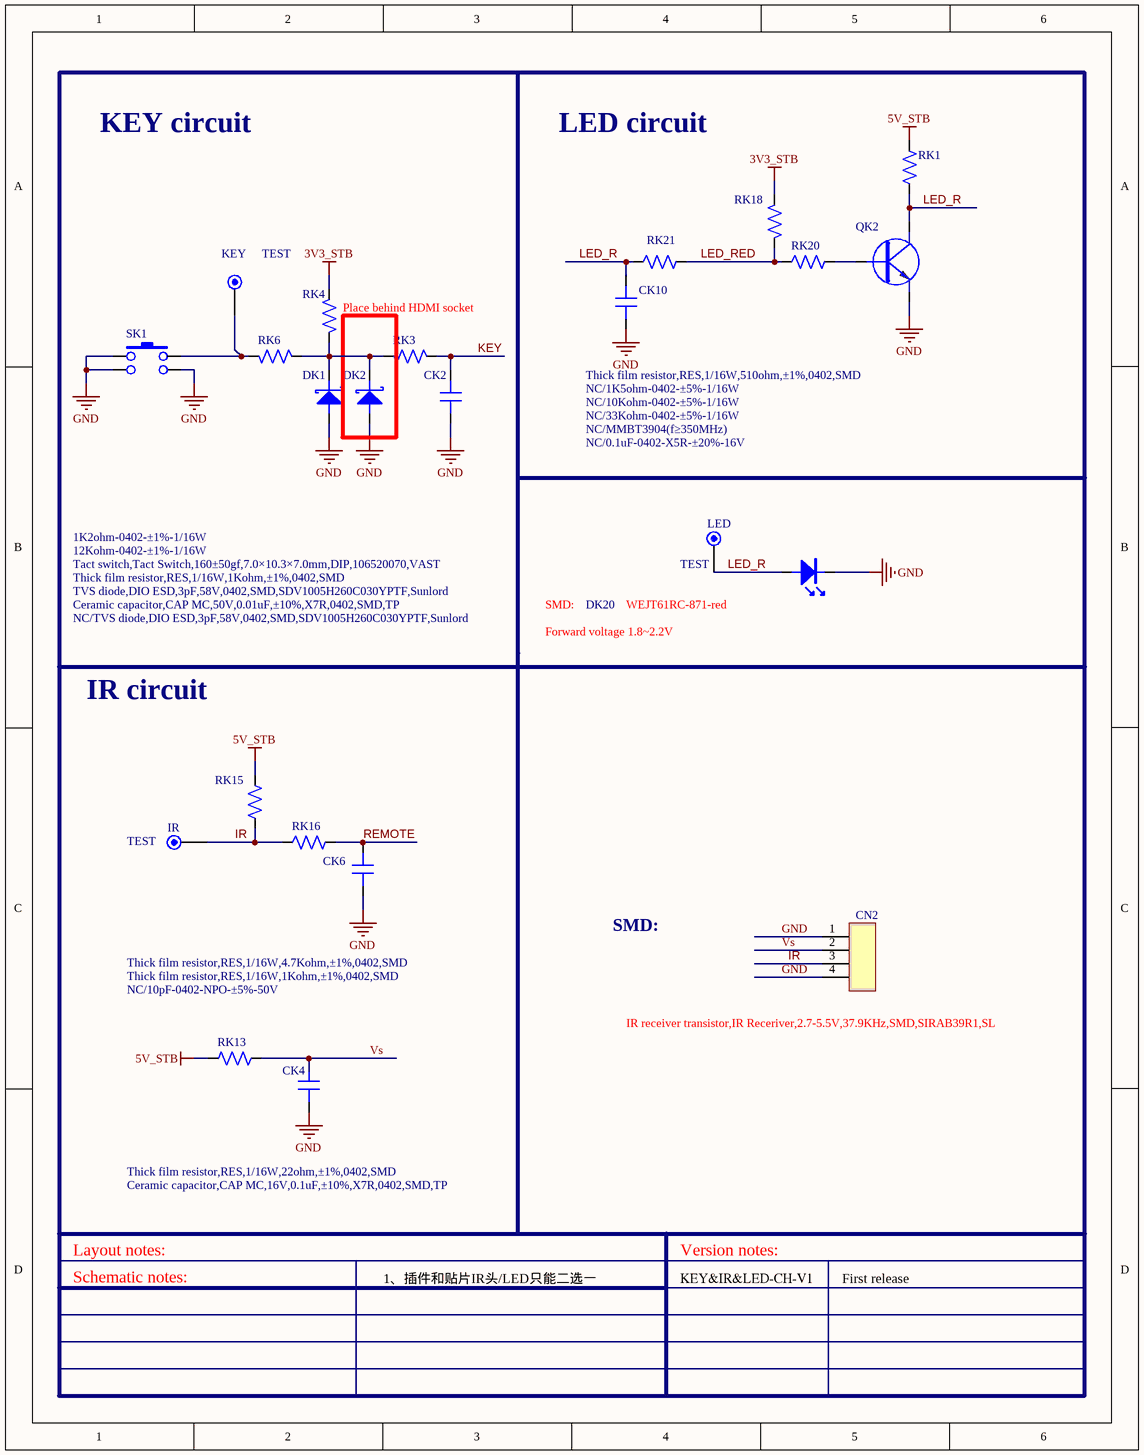
[diagram p0: MISC86383-17.SchDoc]
# Altium schematic sheet MISC86383-17.SchDoc
size 213 x 271 mm

## Parts
CK2  Ceramic capacitor,CAP MC,50V,0.01uF,±10%,X7R,0402,SMD,TP  [C0402]
CK4  Ceramic capacitor,CAP MC,16V,0.1uF,±10%,X7R,0402,SMD,TP  [C0402]
CK6  NC/10pF-0402-NPO-±5%-50V  [C0402]
CK10  NC/0.1uF-0402-X5R-±20%-16V  [C0402]
CN2  IR receiver transistor,IR Receriver,2.7-5.5V,37.9KHz,SMD,SIRAB39R1,SL  [REMOTE-HS-1]
DK1  TVS diode,DIO ESD,3pF,58V,0402,SMD,SDV1005H260C030YPTF,Sunlord  [DIODE-S0402]
DK2  NC/TVS diode,DIO ESD,3pF,58V,0402,SMD,SDV1005H260C030YPTF,Sunlord  [DIODE-S0402]
DK20  WEJT61RC-871-red  [DIODE-S0603]
IR  TEST  [TP]
KEY  TEST  [TP]
LED  TEST  [TP]
QK2  NC/MMBT3904(f≥350MHz)  [SOT-23]
RK1  NC/1K5ohm-0402-±5%-1/16W  [R0402]
RK3  Thick film resistor,RES,1/16W,1Kohm,±1%,0402,SMD  [R0402]
RK4  12Kohm-0402-±1%-1/16W  [R0402]
RK6  1K2ohm-0402-±1%-1/16W  [R0402]
RK13  Thick film resistor,RES,1/16W,22ohm,±1%,0402,SMD  [R0402]
RK15  Thick film resistor,RES,1/16W,4.7Kohm,±1%,0402,SMD  [R0402]
RK16  Thick film resistor,RES,1/16W,1Kohm,±1%,0402,SMD  [R0402]
RK18  NC/33Kohm-0402-±5%-1/16W  [R0402]
RK20  NC/10Kohm-0402-±5%-1/16W  [R0402]
RK21  Thick film resistor,RES,1/16W,510ohm,±1%,0402,SMD  [R0402]
SK1  Tact switch,Tact Switch,160±50gf,7.0×10.3×7.0mm,DIP,106520070,VAST  [KEY-HD-6]

## Blocks framed on the sheet
Place behind HDMI socket: DK2

## Nets
3V3_STB: RK4.2 RK18.2
5V_STB: RK1.2 RK13.1 RK15.1
GND: CK2.2 CK4.2 CK6.1 CK10.1 CN2.1 CN2.4 DK1.A DK2.A DK20.K QK2.E SK1.1 SK1.3 SK1.4
IR: CN2.3 IR.1 RK15.2 RK16.2
KEY: CK2.1 RK3.1
LED_R: CK10.2 DK20.A LED.1 QK2.C RK1.1 RK21.2
LED_RED: RK18.1 RK20.2 RK21.1
REMOTE: CK6.2 RK16.1
Vs: CK4.1 CN2.2 RK13.2
NetDK1_K: DK1.K DK2.K RK3.2 RK4.1 RK6.1
NetKEY_1: KEY.1 RK6.2 SK1.2
NetQK2_B: QK2.B RK20.1

## Notes on the sheet
- KEY circuit
- LED circuit
- SMD:
- Forward voltage 1.8~2.2V
- IR circuit
- Layout notes:
- Version notes:
- Schematic notes:
- 1、插件和贴片IR头/LED只能二选一
- KEY&IR&LED-CH-V1
- First release

## Library data of the parts
CK2 = 0.01uF-0402-X7R-±10%-50V-D
CK4 CK10 = 0.1uF-0402-Y5V-+80%-20%-16V-D
CK6 = 10pF-0402-NPO-±5%-50V-D
CN2 = 红外接收三极管,Phototransistor,NPN,6.8×3×3.2mm,SMD,HS75438D,VISHAY-D
DK1 DK2 = AVLC18S02003-D
DK20 = WEJT61RC-871-红色-D
QK2 = MMBT3904(f≥350MHz)-D-NPN: Q-NPN-#-#-#
RK1 = 22ohm-0402-±5%-1/16W-D
RK3 RK16 RK21 = 1Kohm-0402-±5%-1/16W-D
RK4 RK6 = 4K7ohm-0402-±1%-1/16W-D
RK13 = 100ohm-0402-±5%-1/16W-D
RK15 RK18 = 4K7ohm-0402-±5%-1/16W-D
RK20 = 10Kohm-0402-±5%-1/16W-D
SK1 = 轻触开关,Tact Switch,160±50gf,7.0×10.3×7.0mm,DIP,KFC-A06-E-4-7.5/4(R),YK-DLMI